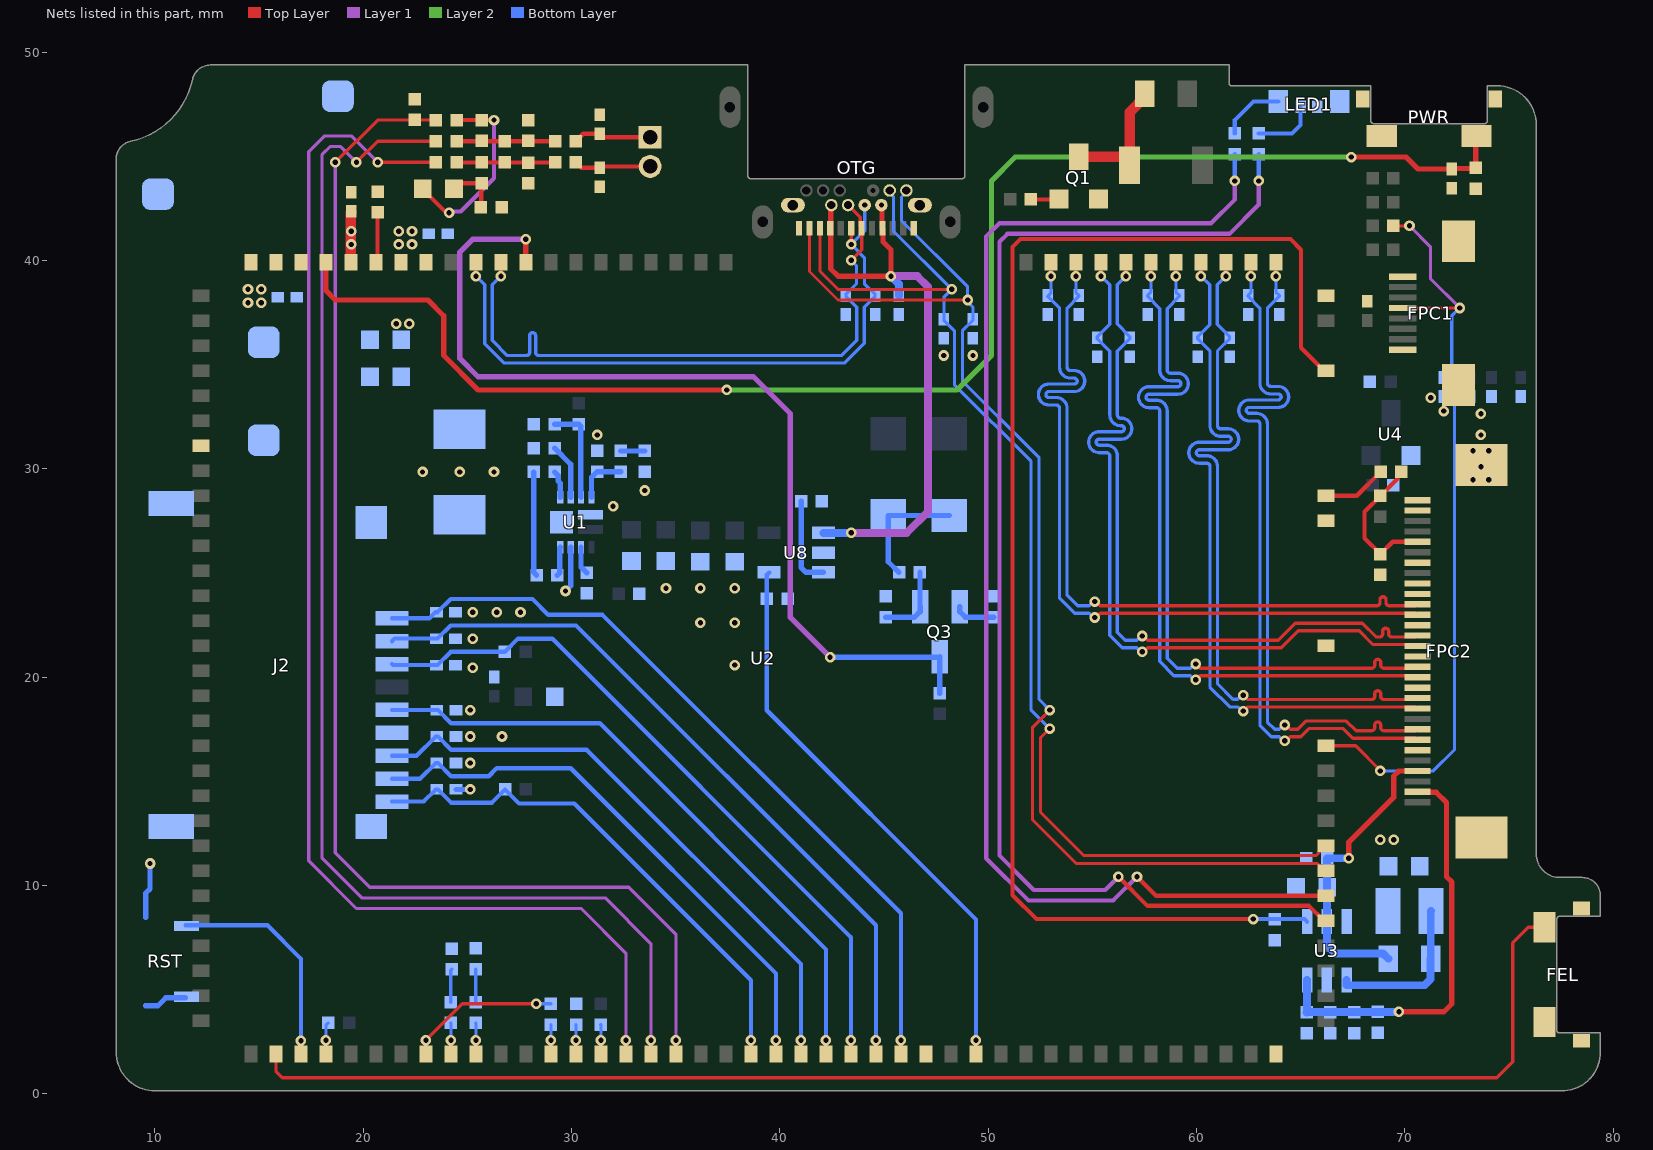
[diagram p0: the nets of this part, all layers, seen from the top]
# Altium PCB MISC105407.PcbDoc (part 2 of 2)
Units mm, origin at the board's own origin, x right, y up, seen from the top; angles counter-clockwise.
Board outline 71.25 x 49.25 mm, 4 copper layers (Top Layer, Layer 1, Layer 2, Bottom Layer), stack 0.603 mm thick; 129 components, 86 nets, 475 pads, 140 vias.

## Via types
v1: diameter 0.508, hole 0.254, Top Layer to Bottom Layer, 140 vias

## Nets (pads, with @x,y where several pads share a name; then routed paths per layer and width w, separated by ;. In a path a pad name is that pad's centre, name@x,y a point inside that pad or via, vN(x,y) a via of type N, cw(c..) or ccw(c..) an arc to the next point about the centre after c; other vN are vias at no path point) (continued)
CTP_TWI1_SDA: ESD7.1 FPC1.5 R5.1 U2.54 | length 37.3
  Top Layer w0.152: U2.54@66.221,16.705 67.642,16.705 68.834,15.513 v1(68.834,15.494) ; R5.1@69.461,41.656 v1(70.231,41.656) ; FPC1.5@69.907,37.715 v1(72.64,37.715)
  Layer 1 w0.152: v1(70.231,41.656) 71.247,40.64 71.247,39.108 v1@72.636,37.719
  Bottom Layer w0.152: v1(68.834,15.494) 71.374,15.494 72.39,16.51 72.39,33.825 71.883,34.331 ESD7.1@71.883,34.382 71.883,34.433 72.061,34.611 72.112,34.611 72.263,34.762 72.263,37.338 v1(72.64,37.715)
GND: C1.1 C3.2 C6.2 C7.2 C8.2 C9.1 C10.1 C11.1 C12.2 C13.1 C14.2 C16.1 C17.1 C18.2 C19.1 C20.2 C21.1 C22.1 C23.1 C27.2 D2.1 D3.2 D5.2 D6.2 D7.2 D8.2 D9.2 D10.2 D11.2 D12.2 D13.2 D14.2 D17.2 D18.1 D19.1 D20.2 D21.2 D22.1 ESD1.2 ESD2.2 ESD5.2 ESD6.2 ESD7.2 ESD8.2 ESD9.2 ESD10.2 ESD11.2 ESD12.2 ESD13.2 ESD14.2 ESD15.2 ESD16.2 ESD17.2 ESD18.2 FEL.1 FEL.3 FEL.4 FPC1.1 FPC1.8 FPC1.9 FPC1.10 FPC2.6 FPC2.12 FPC2.15 FPC2.18 FPC2.21 FPC2.22 FPC2.24 FPC2.29 FPC2.30 FPC2.31 FPC2.32 J2.6 J2.10 J2.11 J2.12 J2.13 LED1.2 LED1.4 OTG.A1 OTG.A12 OTG.B1 OTG.B12 PWR.2 PWR.3 PWR.4 Q1.2 R7.1 R8.1 R10.2 R11.1 R14.2 R15.2 R16.2 R17.2 R18.2 R25.2 R28.2 R29.2 R33.2 R34.1 R38.2 R39.2 R40.2 RST.1 RST.3 RST.4 U1.5 U2.28 U2.42 U2.58 U2.63 U2.72 U2.112 U2.121 U3.2 U4.1 U8.2 VBAT-.1 VIN-.1 | length 5.4
  Bottom Layer w0.254: RST.4@9.566,4.225 10.154,4.225 10.535,4.606 RST.1@11.473,4.606 ; RST.3@9.566,8.475 9.566,9.621 9.779,9.834 v1(9.779,11.049) ; D5.2@24.46,14.605 v1(25.146,14.605)
  other v1: 25.146,15.875 25.146,17.145 26.67,17.145 25.146,18.415 25.273,20.447 37.846,20.574 25.273,21.844 36.195,22.606 37.846,22.606 25.273,23.114 26.416,23.114 27.559,23.114 34.544,24.257 36.195,24.257 37.846,24.257 32.004,28.194 33.528,28.956 73.279,29.464 74.041,29.464 22.86,29.845 24.638,29.845 26.289,29.845 73.66,30.099 73.279,30.861 74.041,30.861 31.242,31.623 73.66,31.623 73.66,32.639 71.882,32.766 71.247,33.401 47.879,35.433 49.276,35.433
HBIAS: R9.1 U2.13 | length 1.4
  Top Layer w0.158: U2.13@29.021,1.905 v1(29.021,2.567)
  Bottom Layer w0.158: R9.1@29.019,3.31 29.021,3.308 v1(29.021,2.567)
HP_DET: R12.2 U2.15 | length 1.4
  Top Layer w0.158: U2.15@31.421,1.905 v1(31.421,2.567)
  Bottom Layer w0.158: R12.2@31.414,3.31 31.421,3.303 v1(31.421,2.567)
HPOUTFB: R8.2 U2.14 | length 1.4
  Top Layer w0.158: U2.14@30.221,1.905 v1(30.221,2.567)
  Bottom Layer w0.158: v1(30.221,2.567) 30.221,3.305 R8.2@30.226,3.31
HS_MIC: R9.2 U2.8 | length 7.4
  Top Layer w0.158: U2.8@23.021,1.905 v1(23.021,2.567) 24.772,4.318 v1(28.321,4.318)
  Bottom Layer w0.158: v1(28.321,4.318) 29.011,4.318 R9.2@29.019,4.31
LCD_PWM: R15.1 U2.69 U3.4 | length 66.3
  Top Layer w0.203: v1(62.738,8.382) 52.324,8.382 51.181,9.525 51.181,40.64 51.562,41.021 64.516,41.021 65.024,40.513 65.024,35.807 66.126,34.705 U2.69@66.221,34.705
  Bottom Layer w0.203: v1(62.738,8.382) 65.193,8.382 U3.4@65.317,8.258
LED1: R26.1 U2.47 | length 62.6
  Top Layer w0.203: v1(56.261,10.414) 57.658,9.017 65.414,9.017 66.126,8.305 U2.47@66.221,8.305
  Layer 1 w0.203: v1(56.261,10.414) 55.626,9.779 52.197,9.779 50.546,11.43 50.546,40.894 50.927,41.275 61.595,41.275 62.992,42.672 v1(62.992,43.815)
  Bottom Layer w0.203: v1(62.992,43.815) R26.1@62.992,45.093
LED2: R31.1 U2.48 | length 62.7
  Top Layer w0.203: v1(57.15,10.414) 58.059,9.505 U2.48@66.221,9.505
  Layer 1 w0.203: v1(57.15,10.414) 56.007,9.271 51.943,9.271 49.911,11.303 49.911,41.148 50.546,41.783 60.706,41.783 61.849,42.926 v1(61.849,43.815)
  Bottom Layer w0.203: v1(61.849,43.815) R31.1@61.849,45.093
LEDA1/2: C6.1 C7.1 D4.2 FPC2.4 U3.5 | length 14.5
  Top Layer w0.254: v1(67.31,11.303) 67.31,12.065 69.469,14.224 69.469,15.24 69.72,15.491 FPC2.4@70.61,15.491
  Bottom Layer w0.381: v1(67.31,11.303) C7.1@66.286,11.303 66.276,11.294 66.276,8.267 U3.5@66.267,8.258 66.267,7.139 66.675,6.731 68.961,6.731 D4.2@69.215,6.477
LEDK1/2: FPC2.2 R14.1 R16.1 R17.1 R18.1 U3.3 | length 20.1
  Top Layer w0.254: v1(69.723,3.937) 71.882,3.937 72.263,4.318 72.263,10.16 72.009,10.414 72.009,13.97 71.511,14.468 70.633,14.468 FPC2.2@70.61,14.491
  Bottom Layer w0.381: R18.1@65.288,3.908 65.303,3.922 65.303,5.444 U3.3@65.317,5.458 ; R18.1@65.303,3.922 69.708,3.922 v1(69.723,3.937)
LRADC: R13.2 U2.4 | length 1.5
  Top Layer w0.158: U2.4@18.221,1.905 v1(18.221,2.567)
  Bottom Layer w0.158: v1(18.221,2.567) 18.221,3.277 R13.2@18.34,3.397
MBIAS: C12.1 R23.2 U2.18 | length 62.5
  Top Layer w0.158: v1(18.669,44.704) 20.701,46.736 R23.2@23.503,46.736 ; U2.18@35.021,1.905 v1(35.021,2.567)
  Layer 1 w0.158: v1(18.669,44.704) 18.669,11.557 20.32,9.906 32.766,9.906 35.021,7.651 v1(35.021,2.567)
MCU_RXD: ESD2.1 OTG.A11 OTG.B11 U2.49 | length 59.4
  Top Layer w0.152: OTG.A11@41.433,41.545 41.433,39.466 42.799,38.1 v1(49.022,38.1) ; v1(52.959,18.415) 52.141,17.597 52.141,13.137 54.229,11.049 65.808,11.049 65.897,10.96 65.897,10.934 66.126,10.705 U2.49@66.221,10.705
  Bottom Layer w0.152: OTG.B11@46.083,43.355 46.083,43.278 45.847,43.042 45.847,41.91 49.022,38.735 v1(49.022,38.1) 49.022,38.004 49.277,37.748 ESD2.1@49.277,37.176 49.277,37.125 48.768,36.616 48.768,34.213 52.451,30.53 52.451,18.923 v1(52.959,18.415)
MCU_TXD: ESD1.1 OTG.A10 OTG.B10 U2.50 | length 57.1
  Top Layer w0.152: OTG.A10@41.933,41.545 41.933,39.474 42.799,38.608 v1(48.26,38.608) ; v1(52.959,17.526) 52.521,17.088 52.521,13.519 54.61,11.43 65.746,11.43 65.897,11.581 65.897,11.676 66.126,11.905 U2.50@66.221,11.905
  Bottom Layer w0.152: OTG.B10@45.283,43.355 45.283,43.234 45.466,43.051 45.466,41.402 v1(48.26,38.608) 47.88,38.228 ESD1.1@47.88,37.176 47.88,37.125 48.387,36.619 48.387,34.036 52.07,30.353 52.07,18.415 v1(52.959,17.526)
MICIN1_N: C26.2 U2.16 | length 62.9
  Top Layer w0.158: v1(20.701,44.704) C26.2@23.503,44.704 ; U2.16@32.621,1.905 v1(32.621,2.567)
  Layer 1 w0.158: v1(20.701,44.704) 19.431,45.974 18.161,45.974 17.399,45.212 17.399,11.176 19.685,8.89 30.48,8.89 32.621,6.749 v1(32.621,2.567)
MICIN1_P: C15.2 U2.17 | length 62.9
  Top Layer w0.158: v1(19.685,44.704) 20.701,45.72 C15.2@23.503,45.72 ; U2.17@33.821,1.905 v1(33.821,2.567)
  Layer 1 w0.158: v1(19.685,44.704) 18.923,45.466 18.415,45.466 18.034,45.085 18.034,11.303 19.939,9.398 31.623,9.398 33.821,7.2 v1(33.821,2.567)
MIPI_CL_N: ESD14.1 FPC2.13 U2.78 | length 35.5
  Top Layer w0.158: v1(57.821,39.243) U2.78@57.821,39.905 ; v1(59.977,19.866) 60.171,20.061 70.541,20.061 FPC2.13@70.61,19.992
  Bottom Layer w0.158: v1(57.821,39.243) 57.821,38.481 ESD14.1@57.659,38.319 57.659,38.268 58.241,37.687 58.241,36.576 58.241,35.433 58.241,34.743 ccw(c58.76,34.743) 58.76,34.223 59.114,34.223 cw(c59.114,34.081) 59.114,33.938 57.729,33.938 ccw(c57.729,33.434) 57.729,32.93 58.082,32.93 cw(c58.082,32.772) 58.241,32.772 58.241,32.512 58.241,32.258 58.241,31.877 58.241,31.623 58.241,20.75 58.924,20.067 59.709,20.067 59.909,19.866 v1(59.977,19.866)
MIPI_CL_P: ESD13.1 FPC2.14 U2.77 | length 35.5
  Top Layer w0.158: v1(59.021,39.243) U2.77@59.021,39.905 ; v1(59.977,20.628) 60.183,20.422 68.326,20.422 68.405,20.422 ccw(c68.405,20.58) 68.563,20.58 68.563,20.706 cw(c68.706,20.706) 68.849,20.706 68.849,20.58 ccw(c69.007,20.58) 69.007,20.422 69.469,20.422 70.541,20.422 FPC2.14@70.61,20.491
  Bottom Layer w0.158: v1(59.021,39.243) 59.021,38.482 ESD13.1@59.183,38.319 59.183,38.268 58.602,37.687 58.602,36.576 58.602,35.433 58.602,34.743 ccw(c58.76,34.743) 58.76,34.585 59.114,34.585 cw(c59.114,34.081) 59.114,33.577 57.729,33.577 ccw(c57.729,33.434) 57.729,33.292 58.082,33.292 cw(c58.082,32.772) 58.602,32.772 58.602,32.512 58.602,32.258 58.602,31.877 58.602,31.623 58.602,20.9 59.074,20.428 59.709,20.428 59.909,20.628 v1(59.977,20.628)
MIPI_D0_N: ESD18.1 FPC2.7 U2.74 | length 34.1
  Top Layer w0.158: v1(62.621,39.243) U2.74@62.621,39.905 ; v1(64.247,16.936) 64.314,16.936 64.515,17.136 65.015,17.136 65.405,17.526 67.053,17.526 67.518,17.061 70.541,17.061 FPC2.7@70.61,16.992
  Bottom Layer w0.158: v1(62.621,39.243) 62.621,38.455 ESD18.1@62.485,38.319 62.485,38.268 63.054,37.7 63.054,35.687 63.054,35.052 63.054,34.108 ccw(c63.573,34.108) 63.573,33.588 63.927,33.588 cw(c63.927,33.446) 63.927,33.303 62.542,33.303 ccw(c62.542,32.799) 62.542,32.295 62.895,32.295 cw(c62.895,32.137) 63.054,32.137 63.054,31.877 63.054,17.688 63.606,17.136 63.979,17.136 64.18,16.936 v1(64.247,16.936)
MIPI_D0_P: ESD17.1 FPC2.8 U2.73 | length 34.1
  Top Layer w0.158: v1(63.821,39.243) U2.73@63.821,39.905 ; v1(64.247,17.698) 64.314,17.698 64.515,17.497 64.865,17.497 65.255,17.887 67.203,17.887 67.668,17.422 68.326,17.422 68.405,17.422 ccw(c68.405,17.58) 68.563,17.58 68.563,17.703 cw(c68.706,17.703) 68.849,17.703 68.849,17.58 ccw(c69.007,17.58) 69.007,17.422 69.596,17.422 70.541,17.422 FPC2.8@70.61,17.491
  Bottom Layer w0.158: v1(63.821,39.243) 63.821,38.481 ESD17.1@63.983,38.319 63.983,38.268 63.415,37.7 63.415,35.687 63.415,35.052 63.415,34.108 ccw(c63.573,34.108) 63.573,33.95 63.927,33.95 cw(c63.927,33.446) 63.927,32.942 62.542,32.942 ccw(c62.542,32.799) 62.542,32.657 62.895,32.657 cw(c62.895,32.137) 63.415,32.137 63.415,31.877 63.415,17.838 63.756,17.497 63.979,17.497 64.18,17.698 v1(64.247,17.698)
MIPI_D1_N: ESD16.1 FPC2.10 U2.76 | length 34.8
  Top Layer w0.158: v1(60.221,39.243) U2.76@60.221,39.905 ; v1(62.247,18.367) 62.441,18.561 70.541,18.561 FPC2.10@70.61,18.491
  Bottom Layer w0.158: v1(60.221,39.243) 60.64,38.824 60.64,36.906 60.072,36.338 ESD16.1@60.072,36.287 60.072,36.236 60.654,35.655 60.654,32.893 60.654,32.076 ccw(c61.173,32.076) 61.173,31.556 61.527,31.556 cw(c61.527,31.414) 61.527,31.271 60.142,31.271 ccw(c60.142,30.767) 60.142,30.263 60.495,30.263 cw(c60.495,30.105) 60.654,30.105 60.654,29.845 60.654,29.721 60.654,19.519 61.606,18.567 61.979,18.567 62.18,18.367 v1(62.247,18.367)
MIPI_D1_P: ESD15.1 FPC2.11 U2.75 | length 34.8
  Top Layer w0.158: v1(61.421,39.243) U2.75@61.421,39.905 ; v1(62.247,19.129) 62.453,18.922 68.326,18.922 68.405,18.922 ccw(c68.405,19.08) 68.563,19.08 68.563,19.2 cw(c68.706,19.2) 68.849,19.2 68.849,19.08 ccw(c69.007,19.08) 69.007,18.922 69.342,18.922 70.541,18.922 FPC2.11@70.61,18.992
  Bottom Layer w0.158: v1(61.421,39.243) 61.002,38.824 61.002,36.933 61.596,36.338 ESD15.1@61.596,36.287 61.596,36.236 61.015,35.655 61.015,32.893 61.015,32.076 ccw(c61.173,32.076) 61.173,31.918 61.527,31.918 cw(c61.527,31.414) 61.527,30.91 60.142,30.91 ccw(c60.142,30.767) 60.142,30.625 60.495,30.625 cw(c60.495,30.105) 61.015,30.105 61.015,29.845 61.015,29.721 61.015,19.669 61.756,18.928 61.979,18.928 62.18,19.129 v1(62.247,19.129)
MIPI_D2_N: ESD12.1 FPC2.16 U2.80 | length 37
  Top Layer w0.158: v1(55.421,39.243) U2.80@55.421,39.905 ; v1(57.404,21.209) 57.471,21.209 57.672,21.409 64.081,21.409 64.895,22.223 67.816,22.223 68.479,21.561 70.541,21.561 FPC2.16@70.61,21.491
  Bottom Layer w0.158: v1(55.421,39.243) 55.84,38.824 55.84,36.932 55.246,36.338 ESD12.1@55.246,36.287 55.246,36.236 55.848,35.634 55.848,34.798 55.848,33.274 55.848,32.584 ccw(c56.368,32.584) 56.368,32.064 56.402,32.064 cw(c56.402,31.922) 56.402,31.779 55.336,31.779 ccw(c55.336,31.275) 55.336,30.771 55.69,30.771 cw(c55.69,30.613) 55.848,30.613 55.848,30.353 55.848,22 56.439,21.409 57.136,21.409 57.337,21.209 v1(57.404,21.209)
MIPI_D2_P: ESD11.1 FPC2.17 U2.79 | length 37
  Top Layer w0.158: v1(56.621,39.243) U2.79@56.621,39.905 ; v1(57.404,21.971) 57.471,21.971 57.672,21.771 63.932,21.771 64.746,22.585 67.966,22.585 68.629,21.922 68.707,21.922 68.786,21.922 ccw(c68.786,22.08) 68.944,22.08 68.944,22.205 cw(c69.087,22.205) 69.23,22.205 69.23,22.08 ccw(c69.388,22.08) 69.388,21.922 69.723,21.922 70.541,21.922 FPC2.17@70.61,21.992
  Bottom Layer w0.158: v1(56.621,39.243) 56.202,38.824 56.202,36.948 56.812,36.338 ESD11.1@56.812,36.287 56.812,36.236 56.21,35.634 56.21,34.798 56.21,33.274 56.21,32.584 ccw(c56.368,32.584) 56.368,32.426 56.402,32.426 cw(c56.402,31.922) 56.402,31.418 55.336,31.418 ccw(c55.336,31.275) 55.336,31.133 55.69,31.133 cw(c55.69,30.613) 56.21,30.613 56.21,30.353 56.21,22.149 56.588,21.771 57.136,21.771 57.337,21.971 v1(57.404,21.971)
MIPI_D3_N: ESD10.1 FPC2.19 U2.82 | length 37
  Top Layer w0.158: v1(53.021,39.243) U2.82@53.021,39.905 ; v1(55.118,22.86) 55.185,22.86 55.386,23.06 62.833,23.06 70.541,23.061 FPC2.19@70.61,22.992
  Bottom Layer w0.158: v1(53.021,39.243) 53.021,38.415 52.874,38.268 53.434,37.709 53.434,35.941 53.434,34.87 ccw(c53.953,34.87) 53.953,34.35 54.137,34.35 cw(c54.137,34.208) 54.137,34.065 52.922,34.065 ccw(c52.922,33.561) 52.922,33.057 53.275,33.057 cw(c53.275,32.899) 53.434,32.899 53.434,32.639 53.434,23.779 54.153,23.06 54.85,23.06 55.051,22.86 v1(55.118,22.86)
MIPI_D3_P: ESD9.1 FPC2.20 U2.81 | length 37
  Top Layer w0.158: v1(54.221,39.243) U2.81@54.221,39.905 ; v1(55.118,23.622) 55.185,23.622 55.386,23.422 62.683,23.422 ; 62.683,23.422 68.58,23.422 68.659,23.422 ccw(c68.659,23.58) 68.817,23.58 68.817,23.71 cw(c68.96,23.71) 69.103,23.71 69.103,23.58 ccw(c69.261,23.58) 69.261,23.422 69.596,23.422 70.541,23.422 FPC2.20@70.61,23.491
  Bottom Layer w0.158: v1(54.221,39.243) 54.221,38.456 ESD9.1@54.357,38.319 54.357,38.268 53.795,37.706 53.795,35.941 53.795,34.87 ccw(c53.953,34.87) 53.953,34.712 54.137,34.712 cw(c54.137,34.208) 54.137,33.704 52.922,33.704 ccw(c52.922,33.561) 52.922,33.419 53.275,33.419 cw(c53.275,32.899) 53.795,32.899 53.795,32.639 53.795,23.929 54.302,23.422 54.85,23.422 55.051,23.622 v1(55.118,23.622)
NetC1_2: C1.2 U1.2 | length 2.7
  Bottom Layer w0.254: C1.2@29.194,30.988 29.968,30.214 U1.2@29.968,28.631
NetC2_1: C2.1 U1.10 | length 1.4
  Bottom Layer w0.254: C2.1@29.329,24.892 29.445,25.008 29.445,26.21 U1.10@29.468,26.233
NetC2_2: C2.2 L2.2 R1.1 U1.11 | length 5
  Bottom Layer w0.254: R1.1@28.194,29.845 28.194,25.027 C2.2@28.329,24.892
NetC3_1: C3.1 D2.2 PWR.1 U2.111 | length 71
  Top Layer w0.254: U2.111@18.221,39.905 18.221,38.548 18.669,38.1 23.114,38.1 23.876,37.338 23.876,35.433 25.527,33.782 v1(37.465,33.782) ; v1(67.437,44.958) 70.071,44.958 70.646,44.383 D2.2@72.264,44.383 72.294,44.413 73.377,44.413 C3.1@73.406,44.442 73.406,45.936 PWR.1@73.446,45.976
  Layer 2 w0.254: v1(37.465,33.782) 48.514,33.782 50.165,35.433 50.165,43.815 51.308,44.958 v1(67.437,44.958)
NetC4_1: C4.1 U2.9 | length 1.5
  Top Layer w0.158: U2.9@24.221,1.905 v1(24.221,2.567)
  Bottom Layer w0.158: C4.1@24.212,3.396 24.221,3.387 v1(24.221,2.567)
NetC4_2: C4.2 R10.1 | length 1.6
  Bottom Layer w0.158: C4.2@24.212,4.396 24.212,5.924 R10.1@24.257,5.969
NetC5_1: C5.1 U2.10 | length 1.5
  Top Layer w0.158: U2.10@25.421,1.905 v1(25.421,2.567)
  Bottom Layer w0.158: C5.1@25.418,3.396 25.421,3.393 v1(25.421,2.567)
NetC5_2: C5.2 R11.2 | length 1.6
  Bottom Layer w0.158: R11.2@25.4,5.977 25.418,5.959 C5.2@25.418,4.396
NetC11_2: C11.2 FPC2.26 R19.2 R20.2 | length 7
  Top Layer w0.203: R20.2@69.842,29.845 69.644,29.647 69.644,29.504 R19.2@68.834,28.694 68.072,27.932 68.072,26.662 C11.2@68.834,25.9 69.425,26.491 FPC2.26@70.61,26.491
NetC14_1: C14.1 C15.1 C24.1 R24.2 R30.1 | length 4.7
  Top Layer w0.203: C15.1@24.503,45.72 R30.1@29.218,45.72
NetC18_1: C18.1 R35.1 U1.4 | length 2.5
  Bottom Layer w0.254: U1.4@30.968,28.631 30.968,29.587 C18.1@31.234,29.853 R35.1@32.377,29.853
NetC20_1: C20.1 R35.2 | length 1.1
  Bottom Layer w0.254: R35.2@32.377,30.853 C20.1@33.52,30.853
NetC24_2: C24.2 C26.1 C27.1 R27.2 R32.1 | length 4.7
  Top Layer w0.203: C26.1@24.503,44.704 R32.1@29.218,44.704
NetC25_1: C25.1 R23.1 R24.1 | length 9.2
  Top Layer w0.203: C25.1@22.872,43.434 22.872,43.409 23.99,42.291 v1(24.13,42.291) ; R23.1@24.503,46.736 R24.1@25.689,46.736 v1(26.289,46.736)
  Layer 1 w0.203: v1(24.13,42.291) 24.181,42.342 24.689,42.342 26.289,43.942 v1(26.289,46.736)
NetC25_2: C25.2 R27.1 R28.1 | length 2.6
  Top Layer w0.203: C25.2@24.372,43.434 24.638,43.7 R27.1@25.689,43.7 25.675,43.687 25.675,42.558 R28.1@25.662,42.545
NetD1_1: D1.1 J1.2 Q1.3 | length 6.3
  Top Layer w0.508: Q1.3@54.356,44.983 56.551,44.983 J1.2@56.797,44.737 ; J1.2@56.797,44.577 J1.2@56.797,44.737 ; D1.1@57.531,48.006 57.531,47.841 56.797,47.107 J1.2@56.797,44.737
NetD4_1: D4.1 L1.2 U3.1 | length 7.7
  Bottom Layer w0.381: U3.1@67.217,5.458 67.217,5.211 67.221,5.207 70.949,5.207 71.247,5.505 D4.1@71.247,6.477 71.253,6.483 71.253,8.757 L1.2@71.259,8.763
NetD15_1: D15.1 D16.1 R37.2 | length 5.9
  Bottom Layer w0.254: R37.2@45.728,25.019 45.212,25.535 D15.1@45.212,27.758 D16.1@48.133,27.758
NetD18_2: D18.2 MIC1.2 R32.2 | length 3.7
  Top Layer w0.203: R32.2@30.218,44.704 30.472,44.45 D18.2@31.369,44.45 31.431,44.512 MIC1.2@33.782,44.512
NetD19_2: D19.2 MIC1.1 R30.2 | length 3.8
  Top Layer w0.203: R30.2@30.218,45.72 30.574,46.076 D19.2@31.369,46.076 31.369,46.064 31.521,45.912 MIC1.1@33.782,45.912
NetFEL_2: FEL.2 U2.2 | length 68.2
  Top Layer w0.158: U2.2@15.821,1.905 15.821,1.07 16.129,0.762 74.422,0.762 75.184,1.524 75.184,7.239 75.935,7.99 FEL.2@76.71,7.99
NetLED1_1: LED1.1 R26.2 | length 3
  Bottom Layer w0.203: R26.2@62.992,46.093 64.597,46.093 65.005,46.501 LED1.1@65.005,47.366
NetLED1_3: LED1.3 R31.2 | length 3.1
  Bottom Layer w0.203: R31.2@61.849,46.093 61.849,46.736 62.743,47.63 LED1.3@63.93,47.63
NetQ1_1: Q1.1 R2.2 | length 1.4
  Top Layer w0.203: R2.2@52.062,42.926 53.378,42.926 Q1.1@53.404,42.951
NetQ3_1: Q3.1 R37.1 R38.1 | length 3.7
  Bottom Layer w0.254: R38.1@45.085,22.868 46.468,22.868 46.741,23.141 Q3.1@46.741,23.368 46.736,23.373 R37.1@46.736,25.027
NetQ3_2: Q3.2 R39.1 | length 2
  Bottom Layer w0.254: Q3.2@48.641,23.368 48.641,23.141 48.914,22.868 R39.1@50.292,22.868
NetR1_2: R1.2 U1.1 | length 1.3
  Bottom Layer w0.254: R1.2@29.194,29.845 29.367,29.672 29.367,29.413 29.468,29.312 U1.1@29.468,28.631
NetR3_1: R3.1 R25.1 U1.3 | length 4.7
  Bottom Layer w0.254: R25.1@29.194,32.131 29.198,32.135 30.341,32.135 R3.1@30.345,32.139 30.445,32.039 30.445,28.654 U1.3@30.468,28.631
NetR7_2: R7.2 U2.109 | length 2.4
  Top Layer w0.203: U2.109@20.621,39.905 20.701,39.985 R7.2@20.701,42.299
NetR33_1: R33.1 U8.3 | length 4.4
  Bottom Layer w0.254: R33.1@41.029,28.448 41.029,25.265 41.27,25.024 U8.3@42.097,25.024
NetR34_2: R34.2 U1.8 | length 1.3
  Bottom Layer w0.254: U1.8@30.468,26.233 30.468,25.277 R34.2@30.734,25.011
NetRST_2: RST.2 U2.3 | length 10.8
  Top Layer w0.203: v1@17.018,2.54 v1(17.021,2.537) U2.3@17.021,1.905
  Bottom Layer w0.203: RST.2@11.475,8.084 15.411,8.084 17.021,6.474 v1(17.021,2.537)
PL11: R20.1 U2.64 | length 3.1
  Top Layer w0.203: U2.64@66.221,28.705 67.702,28.705 R20.1@68.842,29.845
SDC0_CLK: D10.1 J2.5 U2.24 | length 30.6
  Top Layer w0.158: U2.24@42.221,1.905 v1(42.221,2.567)
  Bottom Layer w0.203: J2.5@21.395,18.421 21.401,18.415 D10.1@23.546,18.415 23.597,18.415 24.232,17.78 31.369,17.78 42.221,6.928 v1(42.221,2.567)
SDC0_CMD: D11.1 J2.3 R21.2 U2.25 | length 34.1
  Top Layer w0.158: U2.25@43.421,1.905 v1(43.421,2.567)
  Bottom Layer w0.203: J2.3@21.395,20.621 21.441,20.575 D11.1@23.53,20.575 23.581,20.575 24.214,21.209 R21.2@26.805,21.209 27.44,21.844 29.083,21.844 43.421,7.506 v1(43.421,2.567)
SDC0_D0: D9.1 J2.7 U2.23 | length 28.9
  Top Layer w0.158: U2.23@41.021,1.905 v1(41.021,2.567)
  Bottom Layer w0.203: J2.7@21.395,16.221 22.571,16.221 23.495,17.145 D9.1@23.546,17.145 23.597,17.145 24.232,16.51 30.734,16.51 41.021,6.223 v1(41.021,2.567)
SDC0_D1: D8.1 J2.8 U2.22 | length 27.1
  Top Layer w0.158: U2.22@39.821,1.905 v1(39.821,2.567)
  Bottom Layer w0.203: J2.8@21.395,15.121 22.741,15.121 23.495,15.875 D8.1@23.546,15.875 23.597,15.875 24.232,15.24 26.035,15.24 26.416,15.621 29.972,15.621 39.821,5.772 v1(39.821,2.567)
SDC0_D2: D7.1 J2.1 U2.27 | length 37.8
  Top Layer w0.158: U2.27@45.821,1.905 v1(45.821,2.567)
  Bottom Layer w0.203: J2.1@21.395,22.821 23.184,22.821 23.479,23.115 D7.1@23.53,23.115 23.581,23.115 24.214,23.749 28.131,23.749 28.893,22.987 31.496,22.987 45.821,8.662 v1(45.821,2.567)
SDC0_D3: D12.1 J2.2 U2.26 | length 35.7
  Top Layer w0.158: U2.26@44.621,1.905 v1(44.621,2.567)
  Bottom Layer w0.203: J2.2@21.395,21.721 21.52,21.845 D12.1@23.53,21.845 23.581,21.845 24.214,22.479 30.226,22.479 44.621,8.084 v1(44.621,2.567)
SDC0_DET: D5.1 J2.9 R22.2 U2.21 | length 25.3
  Top Layer w0.158: U2.21@38.621,1.905 v1(38.621,2.567)
  Bottom Layer w0.203: J2.9@21.395,14.021 22.911,14.021 23.495,14.605 D5.1@23.546,14.605 23.597,14.605 24.232,13.97 26.187,13.97 R22.2@26.821,14.604 27.495,13.929 30.14,13.929 38.621,5.448 v1(38.621,2.567)
USB0_N: D13.1 OTG.A7 OTG.B7 U2.105 | length 31.4
  Top Layer w0.158: v1(25.421,39.243) U2.105@25.421,39.905 ; v1(43.434,40.767) OTG.A7@43.433,41.545
  Bottom Layer w0.158: v1(25.421,39.243) 25.84,38.824 25.84,36.006 26.774,35.072 43.11,35.072 44.057,36.019 44.057,37.747 44.578,38.268 D13.1@44.578,38.319 44.578,38.37 44.069,38.879 44.069,40.132 v1(43.434,40.767) 44.083,41.416 OTG.B7@44.083,42.655
USB0_P: D3.1 OTG.A6 OTG.B6 U2.104 | length 31.4
  Top Layer w0.158: v1(26.621,39.243) U2.104@26.621,39.905 ; OTG.B6@43.283,42.655 43.862,42.076 43.862,41.616 OTG.A6@43.933,41.545 43.933,40.504 v1(43.434,40.005)
  Bottom Layer w0.158: v1(26.621,39.243) 26.202,38.824 26.202,36.155 26.924,35.433 27.559,35.433 27.841,35.433 ccw(c27.841,35.591) 27.999,35.591 27.999,36.385 cw(c28.142,36.385) 28.284,36.385 28.284,35.591 ccw(c28.443,35.591) 28.443,35.433 28.807,35.433 30.48,35.433 42.96,35.433 43.696,36.168 43.696,37.754 43.181,38.268 D3.1@43.181,38.319 43.181,38.37 43.688,38.877 43.688,39.737 43.434,39.991 v1(43.434,40.005)
USB_HOST: R29.1 U2.30 U8.4 | length 27.3
  Top Layer w0.158: U2.30@49.421,1.905 v1(49.421,2.567)
  Bottom Layer w0.203: U8.4@39.497,25.024 39.378,24.905 R29.1@39.378,23.749 39.378,18.407 49.421,8.364 v1(49.421,2.567)
USB_ID: Q3.3 R36.2 U2.103 | length 46.1
  Top Layer w0.254: v1(27.813,41.021) 27.813,39.913 U2.103@27.821,39.905
  Layer 1 w0.254: v1(27.813,41.021) 25.273,41.021 24.638,40.386 24.638,35.306 25.527,34.417 38.735,34.417 40.513,32.639 40.513,22.86 v1(42.418,20.955)
  Bottom Layer w0.254: v1(42.418,20.955) Q3.3@47.678,20.955 ; R36.2@47.678,19.229 Q3.3@47.678,20.955 ; Q3.3@47.691,20.968 Q3.3@47.678,20.955
VBAT: D20.1 U2.107 U2.108 VBAT+.1
  other v1: 21.717,40.767 22.352,40.767 21.717,41.402 22.352,41.402
VBUS: D14.1 OTG.A4 OTG.A9 OTG.B4 OTG.B9 U8.1 | length 29
  Top Layer w0.254: OTG.B4@42.483,42.655 42.456,42.628 42.456,41.568 42.426,41.537 42.452,41.511 42.452,39.59 42.799,39.243 v1(45.339,39.243) 45.339,40.513 44.956,40.896 44.956,41.522 OTG.A4@44.933,41.545 44.91,41.568 44.91,42.628 OTG.B9@44.883,42.655
  Layer 1 w0.381: v1(43.434,26.924) 46.101,26.924 47.117,27.94 47.117,38.735 46.609,39.243 v1(45.339,39.243)
  Bottom Layer w0.381: U8.1@42.097,26.924 v1(43.434,26.924) ; v1(45.339,39.243) 45.72,38.862 45.72,38.321 D14.1@45.721,38.319
VCC_PS: C8.1 C16.2 C17.2 D22.2 L1.1 L2.1 U1.9 U2.110 U3.6 | length 4.7
  Top Layer w0.508: U2.110@19.421,39.905 19.421,42.298 19.43,42.307 D22.2@19.43,42.358
  Bottom Layer w0.254: v1(29.718,24.13) 29.968,24.38 U1.9@29.968,26.233
  other v1: 68.834,12.192 69.469,12.192 21.59,36.957 22.225,36.957 19.431,40.767 19.431,41.402
VIN: D17.1 U2.113 U2.114 VIN+.1
  other v1: 14.478,37.973 15.113,37.973 14.478,38.608 15.113,38.608
pads on no net: FPC1.2 FPC2.1 FPC2.3 FPC2.5 FPC2.9 FPC2.23 FPC2.25 OTG.2 OTG.3 OTG.4 OTG.5 OTG.A2 OTG.A3 OTG.A8 OTG.B2 OTG.B3 OTG.B8 U2.1 U2.6 U2.7 U2.11 U2.12 U2.19 U2.20 U2.31 U2.32 U2.33 U2.34 U2.35 U2.36 U2.37 U2.38 U2.39 U2.40 U2.41 U2.43 U2.44 U2.45 U2.46 U2.95 U2.96 U2.97 U2.98 U2.99 U2.100 U2.101 U2.102 U2.106 U2.115 U2.116 U2.117 U2.118 U2.119 U2.120 U2.122 U2.123 U2.124 U2.125 U2.126 U2.127 U2.128 U2.129 U2.130 U2.131 U2.132 U2.133 U2.134 U2.135 U2.136 U2.137 U2.138 U2.139 U2.140 U2.141 U2.142 U2.143 U2.144

## Polygon pours and split planes (outlines as drawn)
GND on Top Layer "GND_L01_P001" (solid, remove dead copper, pour order 1): 5.08,51.689 75.438,51.689 84.074,43.053 84.074,2.54 81.534,0 4.318,0
GND on Layer 1 "GND_L02_P002" (solid, remove dead copper, pour order 2): 5.969,50.546 77.724,50.546 82.55,45.72 82.55,2.286 80.264,0 3.048,0
GND on Bottom Layer "GND_L04_P003" (solid, remove dead copper, pour order 3): 8.509,51.308 76.073,51.308 84.074,43.307 84.074,4.318 79.756,0 6.604,0 2.413,4.191
VCC_PS on Layer 2 "VCC_PS_L03_P004" (solid, remove dead copper, pour order 4): 6.731,52.07 77.597,52.07 84.328,45.339 84.328,4.445 79.883,0 6.096,0 0,6.096

## Keep-outs
Keep-Out Layer:
  circle w0.013: c14.736,43.756 r0.75
  circle w0.013: c64.736,43.756 r0.75
  circle w0.013: c73.776,5.756 r0.75
  lines w0.254: 8.026,2.006 ccw(c10.026,2.006) 10.026,0.006 77.526,0.006 ccw(c77.526,2.006) 79.526,2.006 79.526,3.047 79.527,3.048 77.43,3.048 77.43,8.382 79.526,8.382 79.526,8.383 79.526,9.506 ccw(c78.526,9.506) 78.526,10.506 77.446,10.506 cw(c77.446,11.506) 76.446,11.506 76.446,46.506 ccw(c74.446,46.506) 74.446,48.506 73.748,48.506 73.748,46.732 68.572,46.732 68.572,48.506 61.696,48.506 61.696,49.506 48.761,49.506 48.761,44.055 38.601,44.055 38.601,49.506 12.67,49.506 ccw(c12.67,48.506) 11.692,48.717 cw(c8.027,49.506) 8.816,45.84 ccw(c9.027,44.862) 8.026,44.863 8.026,2.006

## Other copper
Top Layer:
  region net VIN: 14.097,40.513 16.256,40.513 16.256,37.592 14.097,37.592
  region net VBAT: 21.336,41.783 23.495,41.783 23.495,39.37 21.336,39.37
Bottom Layer:
  region net VIN: 14.097,38.989 16.256,38.989 16.256,35.179 14.097,35.179
  region net VBAT: 17.526,49.022 22.098,49.022 23.495,47.625 23.495,39.37 21.336,39.37 21.336,46.228 20.701,46.863 17.526,46.863
  region net VCC_PS: 21.082,37.338 22.86,37.338 22.86,33.147 23.114,32.893 26.289,32.893 26.543,32.639 26.543,31.115 26.289,30.861 22.352,30.861 21.082,32.131
  region net VCC_PS: 68.453,12.573 69.85,12.573 69.85,7.62 69.723,7.493 66.929,7.493 66.929,9.017 68.453,10.541 68.453,12.446
  region net NetC2_2: 23.241,28.829 28.067,28.829 28.829,28.067 30.099,28.067 30.099,26.797 23.241,26.797

## Silkscreen, mask and mechanical layers (free items; w line width, h text height)
Mechanical 35:
  text "D1" at 311.961,46.189 h0.38
  text "D1" at 311.961,46.189 h0.38